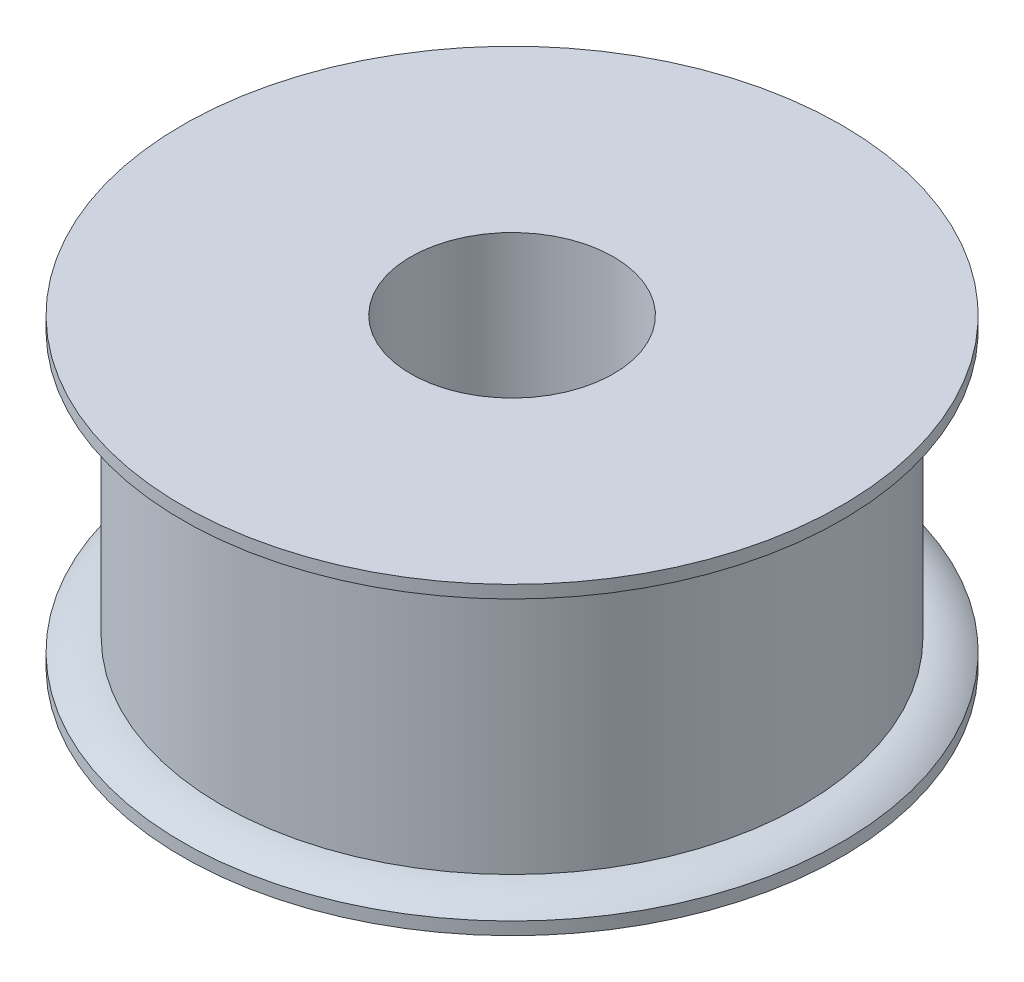
SolidWorks part; units mm, degrees
material "7075-T6"
ref_plane "Front Plane" through (0, 0, 0) normal (0, 0, 1) x (1, 0, 0)
ref_plane "Top Plane" through (0, 0, 0) normal (0, 1, 0) x (1, 0, 0)
ref_plane "Right Plane" through (0, 0, 0) normal (1, 0, 0) x (0, 0, -1)
sketch "Sketch1" plane through (0, 0, 0) normal (0, 0, 1) x (1, 0, 0)
  line L0 (4, 0) -> (11.46, 0) construction
  line L1 (11.46, -5) -> (11.46, 5)
  line L2 (11.46, 5) -> (8, 5)
  line L3 (8, 5) -> (8, 6)
  line L4 (8, 6) -> (4, 6)
  line L5 (4, 6) -> (4, -6)
  line L6 (0, 0) -> (0, 5.5334) construction
  line L7 (8, -6) -> (4, -6)
  line L8 (8, -5) -> (8, -6)
  line L9 (11.46, -5) -> (8, -5)
  dimension "D1" = 22.92
  dimension "D2" = 8
  dimension "D3" = 5
  dimension "D4" = 1
  dimension "D5" = 16
revolve "Revolve1" add sketch "Sketch1" angle 360 about L6
sketch "Sketch2" plane through (0, 0, 0) normal (0, 0, 1) x (1, 0, 0)
  line L0 (8, 6) -> (-8, 6) construction
  line L1 (8, 5) -> (11.46, 5)
  line L2 (8, 5) -> (8, 6)
  line L3 (8, 6) -> (13, 6)
  line L4 (13, 5.5) -> (13, 6)
  line L5 (11.46, -5) -> (11.46, 5) construction
  line L6 (0, 0) -> (0, 8.0995) construction
  line L7 (11.46, 0) -> (14.7966, 0) construction
  line L8 (13, -5.5) -> (13, -6)
  line L9 (8, -6) -> (13, -6)
  line L10 (8, -5) -> (8, -6)
  line L11 (8, -5) -> (11.46, -5)
  arc A0 (11.46, 5) -> (13, 5.5) centre (11.46, 7.6216) ccw
  arc A1 (11.46, -5) -> (13, -5.5) centre (11.46, -7.6216) cw
  dimension "D1" = 0.5
  dimension "D2" = 26
revolve "Revolve2" add sketch "Sketch2" angle 360 about L6
